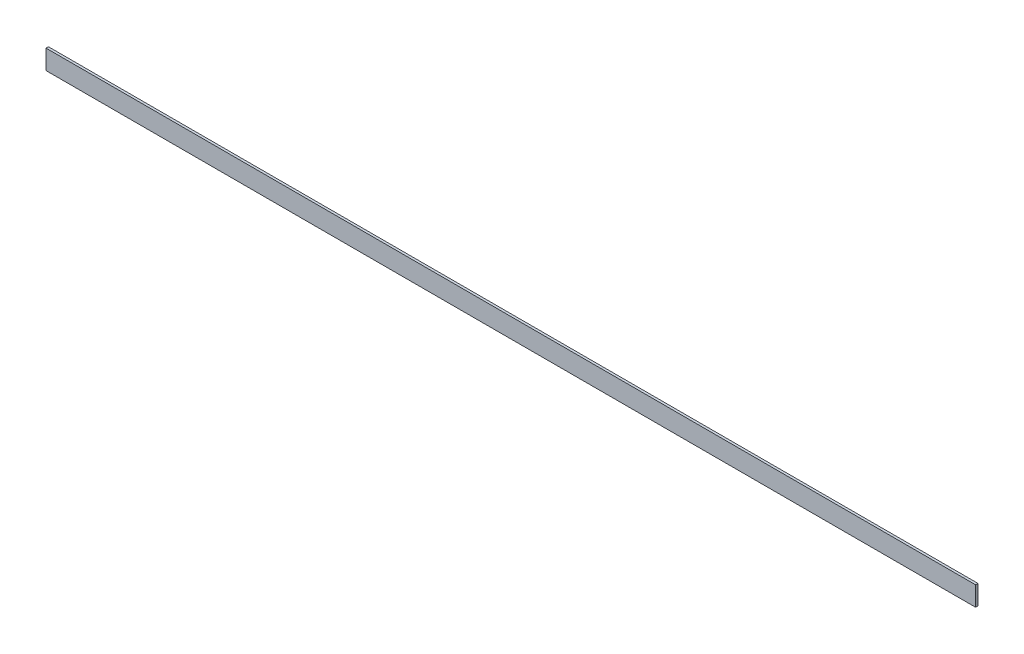
SolidWorks part; units mm, degrees
material "普通碳钢"
ref_plane "Front Plane" through (0, 0, 0) normal (0, 0, 1) x (1, 0, 0)
ref_plane "Top Plane" through (0, 0, 0) normal (0, 1, 0) x (1, 0, 0)
ref_plane "Right Plane" through (0, 0, 0) normal (1, 0, 0) x (0, 0, -1)
sketch "Sketch1" plane through (0, 0, 0) normal (0, 0, 1) x (1, 0, 0)
  line L1 (-1550, -32.5) -> (1550, -32.5)
  line L2 (-1550, -32.5) -> (-1550, 32.5)
  line L3 (-1550, 32.5) -> (1550, 32.5)
  line L4 (1550, -32.5) -> (1550, 32.5)
  line L5 (-1550, -32.5) -> (1550, 32.5) construction
  line L6 (-1550, 32.5) -> (1550, -32.5) construction
  point P0 (0, 0)
  dimension "D1" = 3100
  dimension "D2" = 65
extrude "Boss-Extrude1" add sketch "Sketch1" along normal blind 8
